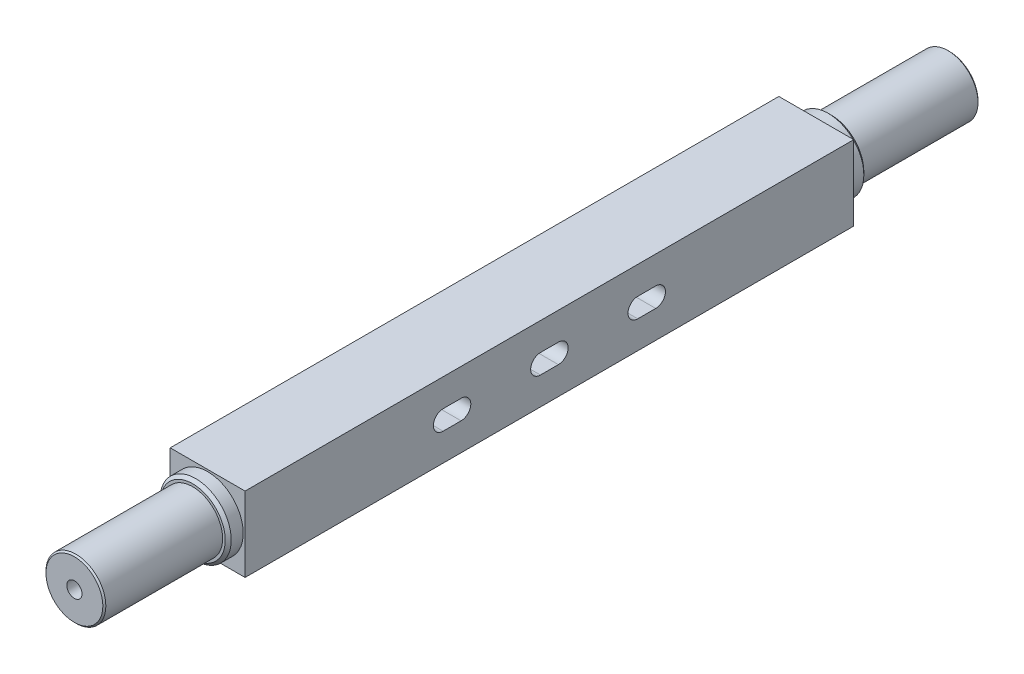
SolidWorks part; units mm, degrees
material "1023 碳钢板 (SS)"
ref_plane "前视基准面" through (0, 0, 0) normal (0, 0, 1) x (1, 0, 0)
ref_plane "上视基准面" through (0, 0, 0) normal (0, 1, 0) x (1, 0, 0)
ref_plane "右视基准面" through (0, 0, 0) normal (1, 0, 0) x (0, 0, -1)
sketch "草图1" plane through (0, 0, 0) normal (0, 0, 1) x (1, 0, 0)
  circle A0 centre (0, 0) radius 20
  dimension "D1" = 40
extrude "凸台-拉伸1" add sketch "草图1" along normal blind 79
sketch "草图2" plane through (0, 0, 79) normal (0, 0, 1) x (1, 0, 0)
  circle A0 centre (0, 0) radius 23.75
  dimension "D1" = 47.5
extrude "凸台-拉伸2" add sketch "草图2" along normal blind 10
chamfer "倒角1" distance 2 angle 45 1 edges at (23.75, 0, 79)
sketch "草图3" plane through (0, 0, 89) normal (0, 0, 1) x (1, 0, 0)
  line L1 (25, 25) -> (-25, 25)
  line L2 (25, 25) -> (25, -25)
  line L3 (25, -25) -> (-25, -25)
  line L4 (-25, 25) -> (-25, -25)
  line L5 (25, 25) -> (-25, -25) construction
  line L6 (25, -25) -> (-25, 25) construction
  point P0 (0, 0)
  dimension "D1" = 50
  dimension "D2" = 50
extrude "凸台-拉伸3" add sketch "草图3" along normal blind 406.5
sketch "草图4" plane through (0, 0, 495.5) normal (0, 0, 1) x (1, 0, 0)
  circle A0 centre (0, 0) radius 23.75
  dimension "D1" = 47.5
extrude "凸台-拉伸4" add sketch "草图4" along normal blind 10
chamfer "倒角2" distance 2 angle 45 1 edges at (23.75, 0, 505.5)
sketch "草图5" plane through (0, 0, 505.5) normal (0, 0, 1) x (1, 0, 0)
  circle A0 centre (0, 0) radius 20
  dimension "D1" = 40
extrude "凸台-拉伸5" add sketch "草图5" along normal blind 79
chamfer "倒角3" distance 1 angle 45 2 edges at (20, 0, 0) (20, 0, 584.5)
hole_wizard "M12 螺纹孔1" positions "草图6" profile "草图7" tap size "M12" standard "ISO"
sketch "草图6" plane through (0, 0, 0) normal (0, 0, -1) x (-1, 0, 0)
  point P0 (0, 0)
sketch "草图7" plane through (0, 0, 0) normal (1, 0, 0) x (0, 1, 0)
  line L0 (0, 0) -> (0, 32.3144)
  line L1 (0, 32.3144) -> (5.1, 29.25)
  line L2 (5.1, 29.25) -> (5.1, 0)
  line L5 (5.1, 0) -> (0, 0)
  line L10 (0, 32.3144) -> (-5.1, 29.25) construction
  line L11 (0, -6.35) -> (0, 107.95) construction
  dimension "螺纹孔钻头直径" = 10.2
  dimension "螺纹孔钻头深度" = 29.25
  dimension "导头角度" = 118
cosmetic thread "孔螺蚊线1" parameters "D1"=24, "D2"=12
hole_wizard "M12 螺纹孔2" positions "草图8" profile "草图9" tap size "M12" standard "ISO"
sketch "草图8" plane through (0, 0, 584.5) normal (0, 0, 1) x (1, 0, 0)
  point P0 (0, 0)
sketch "草图9" plane through (0, 0, 584.5) normal (1, 0, 0) x (0, -1, 0)
  line L0 (0, 0) -> (0, 32.3144)
  line L1 (0, 32.3144) -> (5.1, 29.25)
  line L2 (5.1, 29.25) -> (5.1, 0)
  line L5 (5.1, 0) -> (0, 0)
  line L10 (0, 32.3144) -> (-5.1, 29.25) construction
  line L11 (0, -6.35) -> (0, 107.95) construction
  dimension "螺纹孔钻头直径" = 10.2
  dimension "螺纹孔钻头深度" = 29.25
  dimension "导头角度" = 118
cosmetic thread "孔螺蚊线2" parameters "D1"=24, "D2"=12
sketch "草图10" plane through (25, 0, 0) normal (1, 0, 0) x (0, 0, -1)
  line L0 (-363.25, 0) -> (-351.25, 0) construction
  line L1 (-363.25, 6.5) -> (-351.25, 6.5)
  line L2 (-363.25, -6.5) -> (-351.25, -6.5)
  line L3 (-298.25, 0) -> (-286.25, 0) construction
  line L4 (-298.25, 6.5) -> (-286.25, 6.5)
  line L5 (-298.25, -6.5) -> (-286.25, -6.5)
  line L6 (-233.25, 0) -> (-221.25, 0) construction
  line L7 (-233.25, 6.5) -> (-221.25, 6.5)
  line L8 (-233.25, -6.5) -> (-221.25, -6.5)
  line L9 (-495.5, 25) -> (-89, 25) construction
  arc A0 (-363.25, 6.5) -> (-363.25, -6.5) centre (-363.25, 0) ccw
  arc A1 (-351.25, -6.5) -> (-351.25, 6.5) centre (-351.25, 0) ccw
  arc A2 (-298.25, 6.5) -> (-298.25, -6.5) centre (-298.25, 0) ccw
  arc A3 (-286.25, -6.5) -> (-286.25, 6.5) centre (-286.25, 0) ccw
  arc A4 (-233.25, 6.5) -> (-233.25, -6.5) centre (-233.25, 0) ccw
  arc A5 (-221.25, -6.5) -> (-221.25, 6.5) centre (-221.25, 0) ccw
  point P2 (-357.25, 0)
  point P7 (-292.25, 0)
  point P14 (-227.25, 0)
  point P21 (0, 0)
  point P22 (0, 0)
  point P25 (0, 0)
  point P26 (-292.25, 25)
  dimension "D2" = 6.5
  dimension "D1" = 12
  dimension "D3" = 25
  dimension "D4" = 130
  dimension "D5" = 65
extrude "切除-拉伸1" cut sketch "草图10" against normal blind 79
